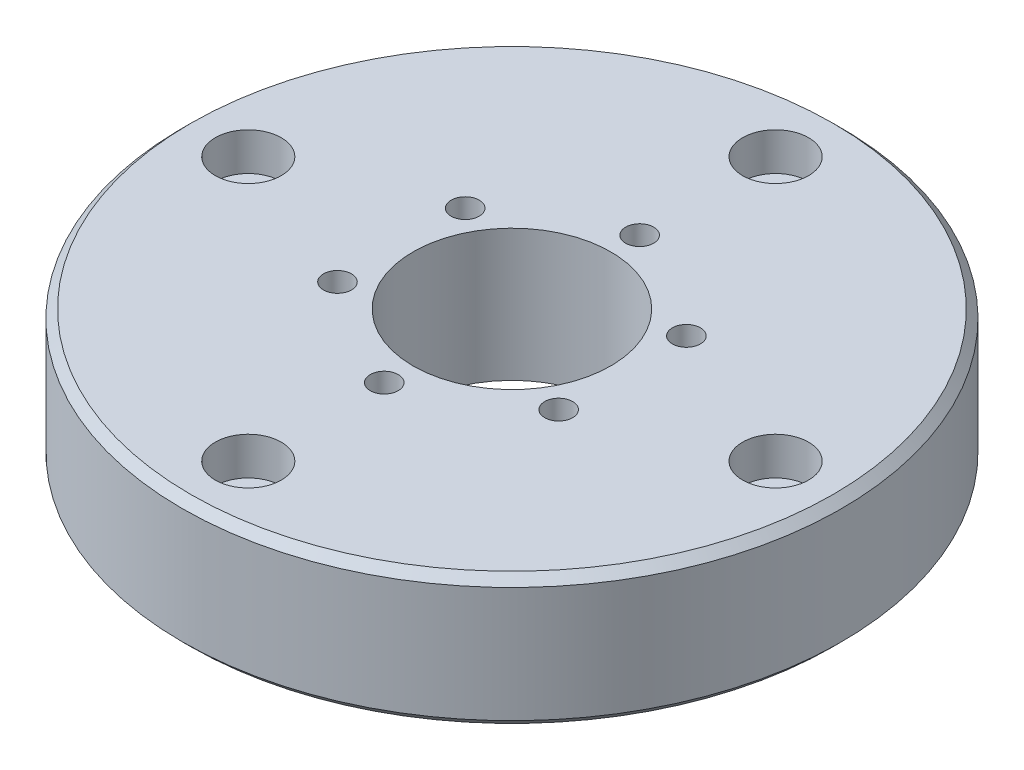
SolidWorks part; units mm, degrees
ref_plane "Front Plane" through (0, 0, 0) normal (0, 0, 1) x (1, 0, 0)
ref_plane "Top Plane" through (0, 0, 0) normal (0, 1, 0) x (1, 0, 0)
ref_plane "Right Plane" through (0, 0, 0) normal (1, 0, 0) x (0, 0, -1)
sketch "Sketch1" plane through (0, 0, 0) normal (0, 1, 0) x (1, 0, 0)
  circle A0 centre (0, 0) radius 40
  circle A1 centre (0, 0) radius 12
  dimension "D1" = 80
  dimension "D2" = 24
extrude "Boss-Extrude1" add sketch "Sketch1" along normal blind 16
sketch "Sketch2" plane through (0, 0, 0) normal (0, -1, 0) x (1, 0, 0)
  point P0 (13.4234, -7.75)
  point P1 (13.4234, 7.75)
  point P3 (0, 15.5)
  point P5 (-13.4234, 7.75)
  point P7 (-13.4234, -7.75)
  point P9 (0, -15.5)
hole_wizard "Hole size (%based) hex socket head cap screw type 1" positions "Sketch3" profile "Sketch4" counterbore size "M3" standard "GB" end condition through all
sketch "Sketch3" plane through (0, 0, 0) normal (0, -1, 0) x (-1, 0, 0)
  point P0 (0, -15.5)
sketch "Sketch4" plane through (0, 0, 15.5) normal (1, 0, 0) x (0, 0, -1)
  line L0 (0, 0) -> (0, 16)
  line L1 (0, 16) -> (1.7, 16)
  line L3 (1.7, 16) -> (1.7, 3.4)
  line L4 (1.7, 3.4) -> (3, 3.4)
  line L5 (3, 3.4) -> (3, 0)
  line L7 (3, 0) -> (0, 0)
  line L11 (0, -6.35) -> (0, 107.95) construction
  dimension "通孔孔直径" = 3.4
  dimension "通孔孔深度" = 16
  dimension "柱形沉头孔直径" = 6
  dimension "柱形沉头孔深度" = 3.4
pattern_sketch "SketchPattern1" of "Hole size (%based) hex socket head cap screw type 1" driven by "Sketch2"
sketch "Sketch5" plane through (0, 16, 0) normal (0, 1, 0) x (1, 0, 0)
  circle A0 centre (0, 0) radius 32 construction
  point P3 (0, 32)
  dimension "D1" = 64
hole_wizard "Hole size (%based) hex socket head cap screw type 2" positions "Sketch6" profile "Sketch7" counterbore size "M4" standard "GB" end condition through all
sketch "Sketch6" plane through (0, 16, 0) normal (0, 1, 0) x (1, 0, 0)
  point P0 (0, 32)
sketch "Sketch7" plane through (0, 16, -32) normal (1, 0, 0) x (0, 0, 1)
  line L0 (0, 0) -> (0, 16)
  line L1 (0, 16) -> (2.25, 16)
  line L3 (2.25, 16) -> (2.25, 4.6)
  line L4 (2.25, 4.6) -> (4, 4.6)
  line L5 (4, 4.6) -> (4, 0)
  line L7 (4, 0) -> (0, 0)
  line L11 (0, -6.35) -> (0, 107.95) construction
  dimension "通孔孔直径" = 4.5
  dimension "通孔孔深度" = 16
  dimension "柱形沉头孔直径" = 8
  dimension "柱形沉头孔深度" = 4.6
pattern_circular "CirPattern1" count 4 over 360 about axis through (0, 0, 0) along (0, 1, 0) of "Hole size (%based) hex socket head cap screw type 2"
chamfer "Chamfer1" distance 1 angle 45 2 edges at (0, 0, 40) (0, 16, 40)
